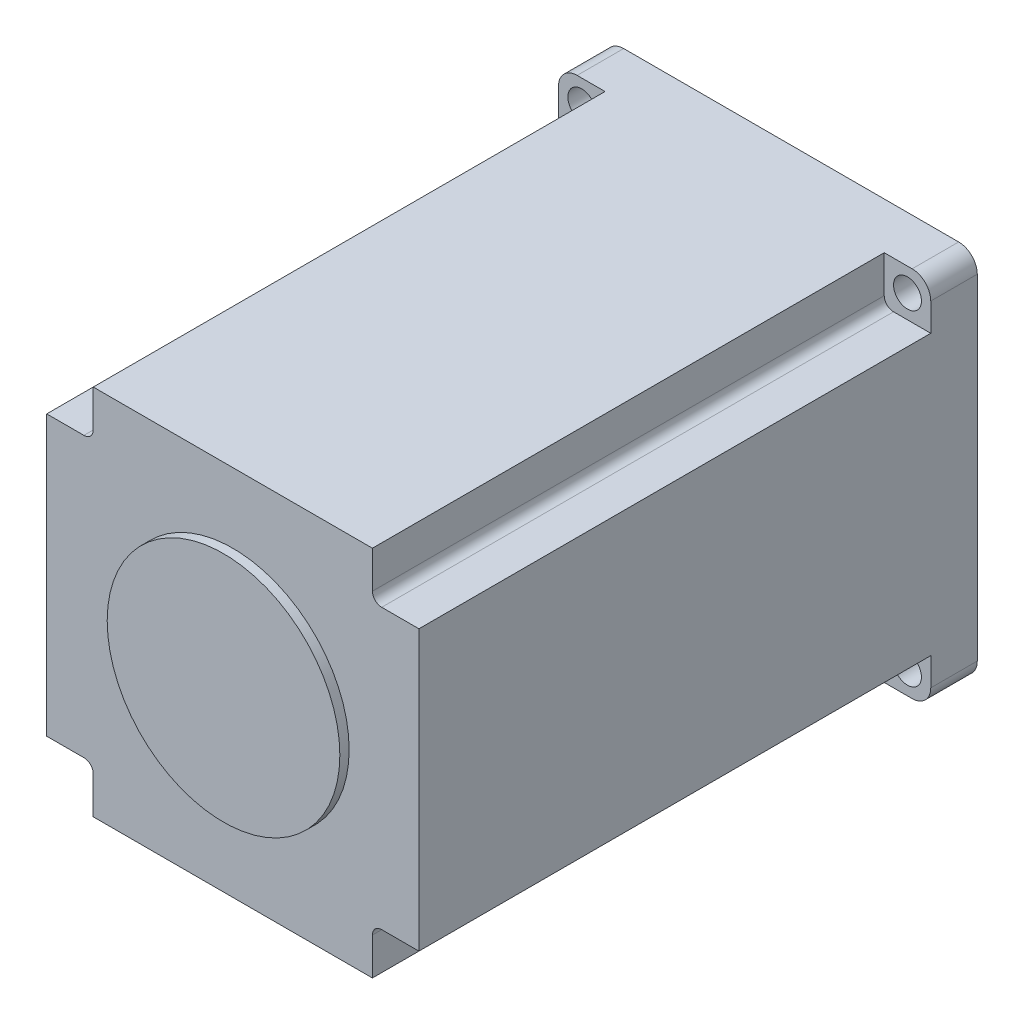
from build123d import *

# Parameters (mm, degrees)
SKETCH1_W           = 40
SKETCH1_H           = 40
BOSS_EXTRUDE1_DEPTH = 30
SKETCH2_W           = 5
SKETCH2_H           = 5
CUT_EXTRUDE1_DEPTH  = 55
SKETCH3_R           = 1.5
CUT_EXTRUDE2_DEPTH  = 55
FILLET1_R           = 2
SKETCH4_R           = 12.5
BOSS_EXTRUDE2_DEPTH = 1
FILLET2_R           = 1
SKETCH5_R           = 5
BOSS_EXTRUDE3_DEPTH = 15


with BuildPart() as part:
    # Sketch1 → Boss-Extrude1 (new, symmetric)
    with BuildSketch(Plane.XY):
        Rectangle(SKETCH1_W, SKETCH1_H)
    extrude(amount=BOSS_EXTRUDE1_DEPTH, both=True)

    # Sketch2 → Cut-Extrude1 (cut)
    with BuildSketch(Plane.XY.offset(30)):
        with Locations((-17.5, 17.5)):
            Rectangle(SKETCH2_W, SKETCH2_H)
        with Locations((17.5, 17.5)):
            Rectangle(SKETCH2_W, SKETCH2_H)
        with Locations((17.5, -17.5)):
            Rectangle(SKETCH2_W, SKETCH2_H)
        with Locations((-17.5, -17.5)):
            Rectangle(SKETCH2_W, SKETCH2_H)
    extrude(amount=-CUT_EXTRUDE1_DEPTH, mode=Mode.SUBTRACT)

    # Sketch3 → Cut-Extrude2 (cut)
    with BuildSketch(Plane.XY.offset(-25)):
        with Locations((-17.5, 17.5)):
            Circle(SKETCH3_R)
        with Locations((17.5, 17.5)):
            Circle(SKETCH3_R)
        with Locations((17.5, -17.5)):
            Circle(SKETCH3_R)
        with Locations((-17.5, -17.5)):
            Circle(SKETCH3_R)
    extrude(amount=-CUT_EXTRUDE2_DEPTH, mode=Mode.SUBTRACT)

    # Fillet1
    fillet1_edges = [part.edges().sort_by_distance(p)[0] for p in [
        (20, -20, -27.5),
        (-20, -20, -27.5),
        (-20, 20, -27.5),
        (20, 20, -27.5),
    ]]
    fillet(fillet1_edges, radius=FILLET1_R)

    # Sketch4 → Boss-Extrude2 (add, symmetric)
    with BuildSketch(Plane.XY.offset(30)):
        Circle(SKETCH4_R)
    extrude(amount=BOSS_EXTRUDE2_DEPTH, both=True)

    # Fillet2
    fillet2_edges = [part.edges().sort_by_distance(p)[0] for p in [
        (-15, -15, 2.5),
        (15, -15, 2.5),
        (15, 15, 2.5),
        (-15, 15, 2.5),
    ]]
    fillet(fillet2_edges, radius=FILLET2_R)

    # Sketch5 → Boss-Extrude3 (add)
    with BuildSketch(Plane(origin=(0, 0, -30), x_dir=(-1, 0, 0), z_dir=(0, 0, -1))):
        with Locations(Location((0, 0, 0), (0, 0, 180))):
            Circle(SKETCH5_R)
    extrude(amount=BOSS_EXTRUDE3_DEPTH)


solid = part.part
